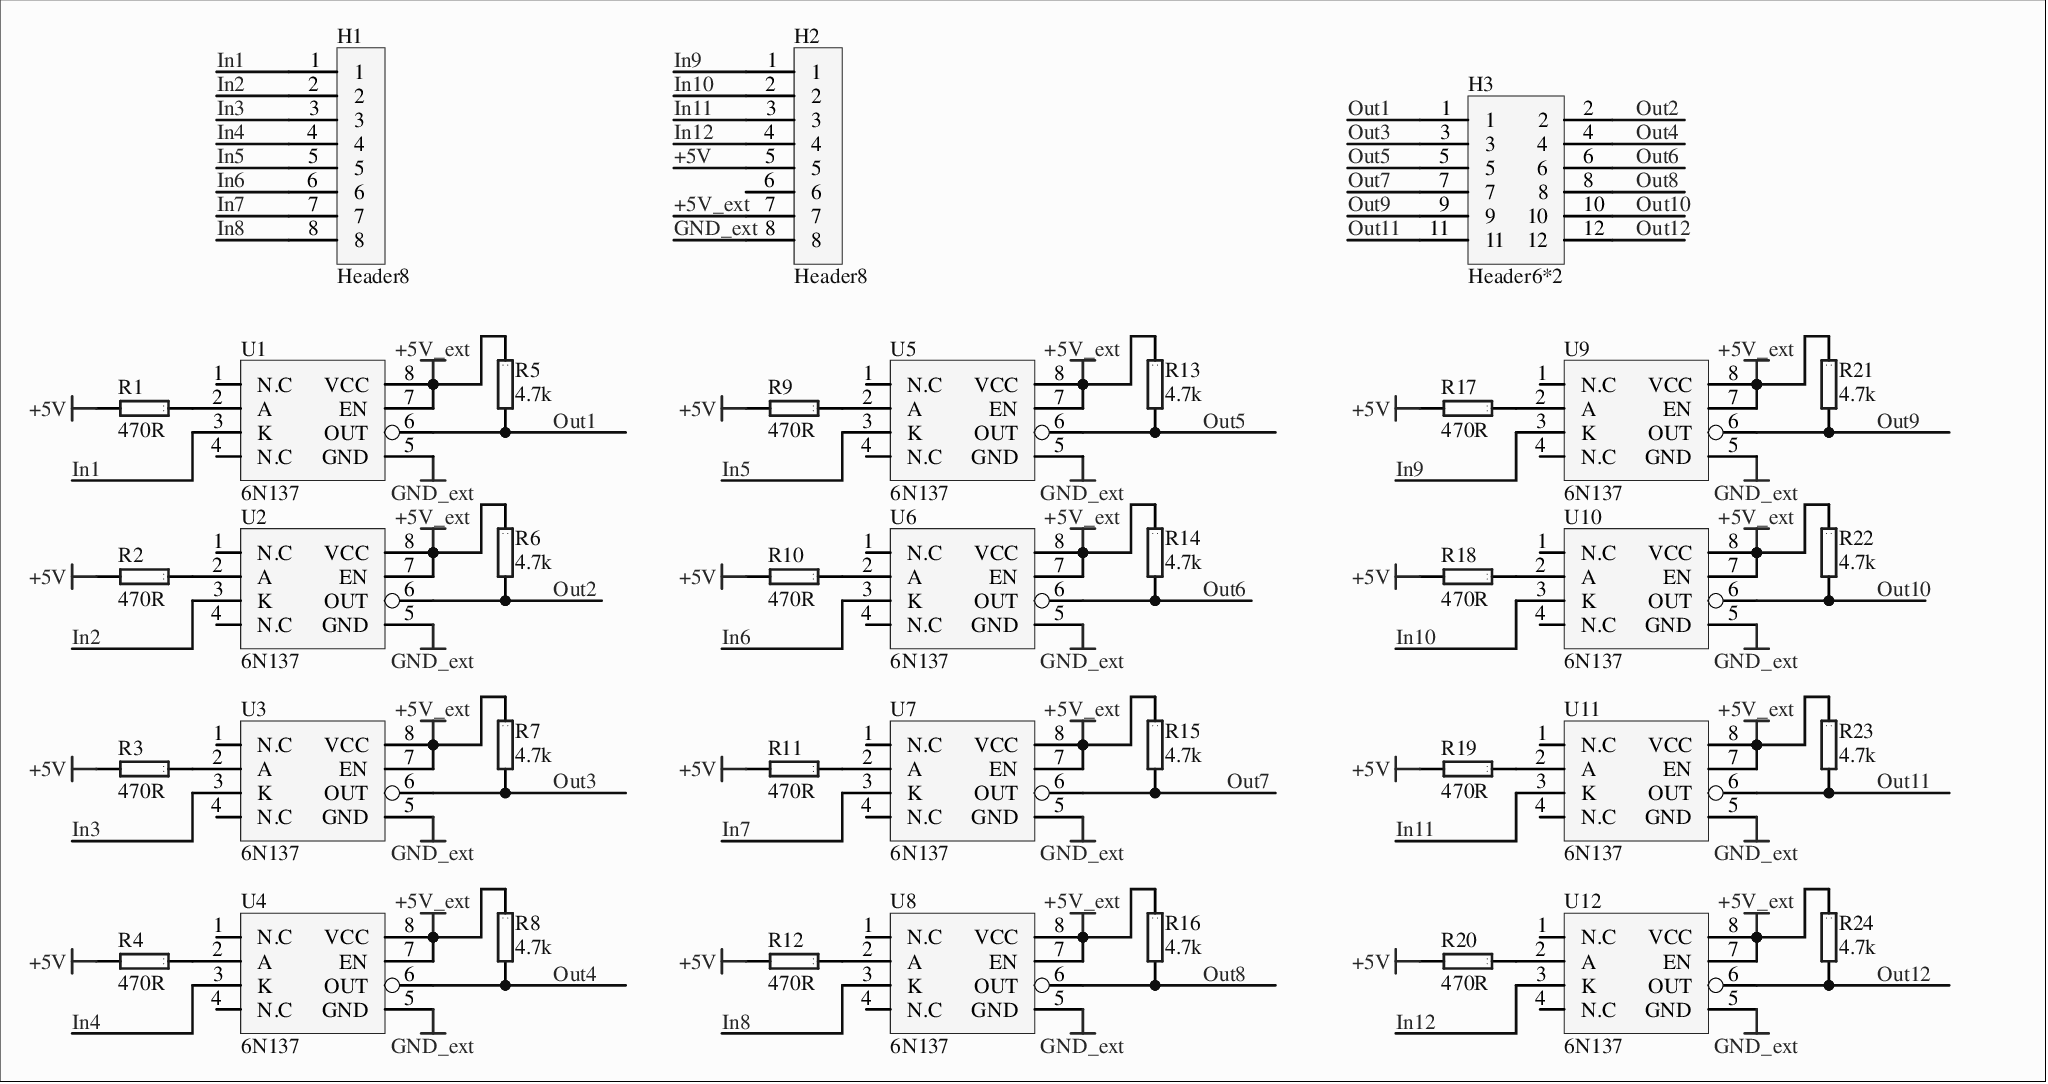
[diagram p0: MISC82214-3.SchDoc]
# Altium project MISC82214-2.PrjPcb
1 sheet, 39 parts. Net scope: global (net labels, ports and power ports of the same name join across sheets).
Board file: MISC82214.PcbDoc

## Sheet MISC82214-3.SchDoc
size 215 x 114 mm

### Parts
H1  Header8  [PinHeader8_1.27mm]
H2  Header8  [PinHeader8_1.27mm]
H3  Header6*2  [PinHeader6*2_2.54mm]
R1  470R  [0603]
R2  470R  [0603]
R3  470R  [0603]
R4  470R  [0603]
R5  4.7k  [0603]
R6  4.7k  [0603]
R7  4.7k  [0603]
R8  4.7k  [0603]
R9  470R  [0603]
R10  470R  [0603]
R11  470R  [0603]
R12  470R  [0603]
R13  4.7k  [0603]
R14  4.7k  [0603]
R15  4.7k  [0603]
R16  4.7k  [0603]
R17  470R  [0603]
R18  470R  [0603]
R19  470R  [0603]
R20  470R  [0603]
R21  4.7k  [0603]
R22  4.7k  [0603]
R23  4.7k  [0603]
R24  4.7k  [0603]
U1  6N137  [6N137_SMD]
U2  6N137  [6N137_SMD]
U3  6N137  [6N137_SMD]
U4  6N137  [6N137_SMD]
U5  6N137  [6N137_SMD]
U6  6N137  [6N137_SMD]
U7  6N137  [6N137_SMD]
U8  6N137  [6N137_SMD]
U9  6N137  [6N137_SMD]
U10  6N137  [6N137_SMD]
U11  6N137  [6N137_SMD]
U12  6N137  [6N137_SMD]

### Nets
+5V: H2.5 R1.2 R2.2 R3.2 R4.2 R9.2 R10.2 R11.2 R12.2 R17.2 R18.2 R19.2 R20.2
+5V_ext: H2.7 R5.1 R6.1 R7.1 R8.1 R13.1 R14.1 R15.1 R16.1 R21.1 R22.1 R23.1 R24.1 U1.7(EN) U1.8(VCC) U2.7(EN) U2.8(VCC) U3.7(EN) U3.8(VCC) U4.7(EN) U4.8(VCC) U5.7(EN) U5.8(VCC) U6.7(EN) U6.8(VCC) U7.7(EN) U7.8(VCC) U8.7(EN) U8.8(VCC) U9.7(EN) U9.8(VCC) U10.7(EN) U10.8(VCC) U11.7(EN) U11.8(VCC) U12.7(EN) U12.8(VCC)
GND_ext: H2.8 U1.5(GND) U2.5(GND) U3.5(GND) U4.5(GND) U5.5(GND) U6.5(GND) U7.5(GND) U8.5(GND) U9.5(GND) U10.5(GND) U11.5(GND) U12.5(GND)
In1: H1.1 U1.3(K)
In2: H1.2 U2.3(K)
In3: H1.3 U3.3(K)
In4: H1.4 U4.3(K)
In5: H1.5 U5.3(K)
In6: H1.6 U6.3(K)
In7: H1.7 U7.3(K)
In8: H1.8 U8.3(K)
In9: H2.1 U9.3(K)
In10: H2.2 U10.3(K)
In11: H2.3 U11.3(K)
In12: H2.4 U12.3(K)
Out1: H3.1 R5.2 U1.6(OUT)
Out2: H3.2 R6.2 U2.6(OUT)
Out3: H3.3 R7.2 U3.6(OUT)
Out4: H3.4 R8.2 U4.6(OUT)
Out5: H3.5 R13.2 U5.6(OUT)
Out6: H3.6 R14.2 U6.6(OUT)
Out7: H3.7 R15.2 U7.6(OUT)
Out8: H3.8 R16.2 U8.6(OUT)
Out9: H3.9 R21.2 U9.6(OUT)
Out10: H3.10 R22.2 U10.6(OUT)
Out11: H3.11 R23.2 U11.6(OUT)
Out12: H3.12 R24.2 U12.6(OUT)
NetR1_1: R1.1 U1.2(A)
NetR2_1: R2.1 U2.2(A)
NetR3_1: R3.1 U3.2(A)
NetR4_1: R4.1 U4.2(A)
NetR9_1: R9.1 U5.2(A)
NetR10_1: R10.1 U6.2(A)
NetR11_1: R11.1 U7.2(A)
NetR12_1: R12.1 U8.2(A)
NetR17_1: R17.1 U9.2(A)
NetR18_1: R18.1 U10.2(A)
NetR19_1: R19.1 U11.2(A)
NetR20_1: R20.1 U12.2(A)

Not connected (* = marked no-connect by the designer): H2 6*; U1 1(N.C) 4(N.C); U2 1(N.C) 4(N.C); U3 1(N.C) 4(N.C); U4 1(N.C) 4(N.C); U5 1(N.C) 4(N.C); U6 1(N.C) 4(N.C); U7 1(N.C) 4(N.C); U8 1(N.C) 4(N.C); U9 1(N.C) 4(N.C); U10 1(N.C) 4(N.C); U11 1(N.C) 4(N.C); U12 1(N.C) 4(N.C)

### Library data of the parts
R1-R24 = RES
U1-U12 = 6N137: High-speed optocoupler